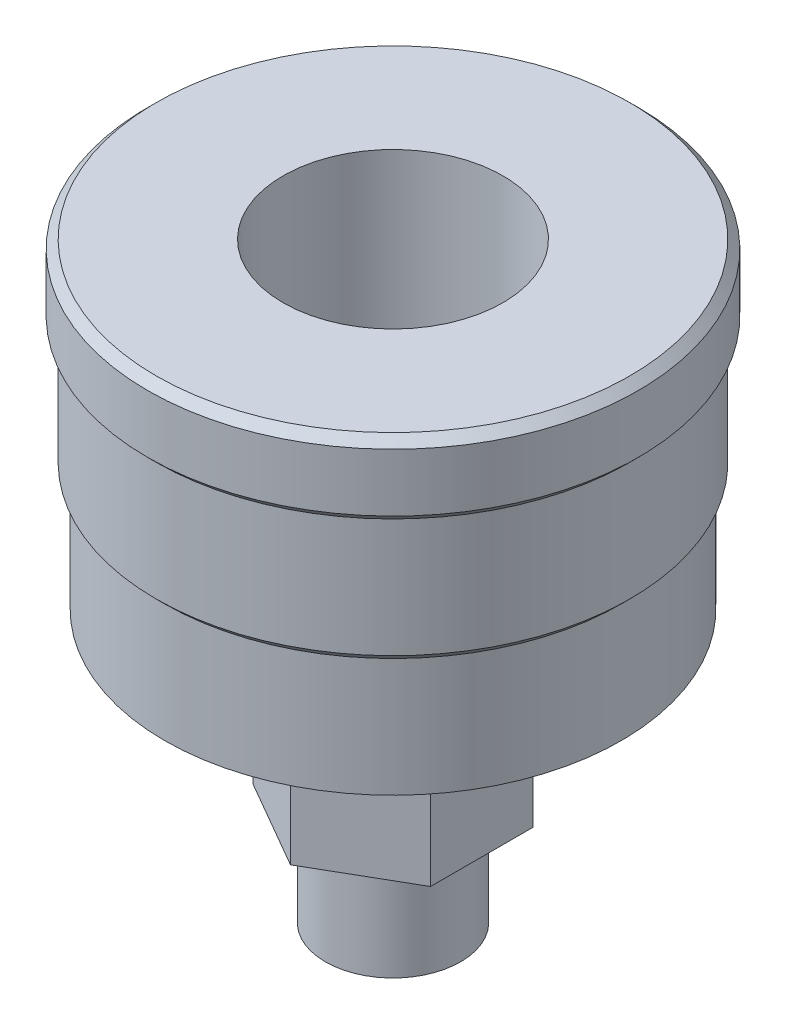
from build123d import *

# Parameters (mm, degrees)
EXTRUDE1_DEPTH = 20.153009


with BuildPart() as part:
    # Sketch1 → Revolve1 (revolve)
    with BuildSketch(Plane.XY, mode=Mode.PRIVATE) as revolve1_sk:
        Polygon((-28, 70), (-29, 69), (-29, 62.153009304), (-28, 61.153009304), (-28, 47.153009304), (-27, 46.153009304), (-27, 32.153009304), (-25, 32.153009304), (-10.5, 22), (-10.5, 12), (-8, 10.698582374), (-8, 0), (-2.5, 0), (-2.5, 32.153009304), (-13.003113073, 47.153009304), (-13.003113073, 70), align=None)
    revolve(revolve1_sk.sketch.rotate(Axis((0, 0, 0), (0, -1, 0)), 270), axis=Axis((0, 0, 0), (0, -1, 0)))

    # Sketch2 → Extrude1 (add)
    with BuildSketch(Plane(origin=(0, 12, 0), x_dir=(-1, 0, 0), z_dir=(0, 1, 0))):
        Polygon((-10.5, 6.062177826), (-10.5, -6.062177826), (0, -12.124355653), (10.5, -6.062177826), (10.5, 6.062177826), (0, 12.124355653), align=None)
    extrude(amount=EXTRUDE1_DEPTH)


solid = part.part
